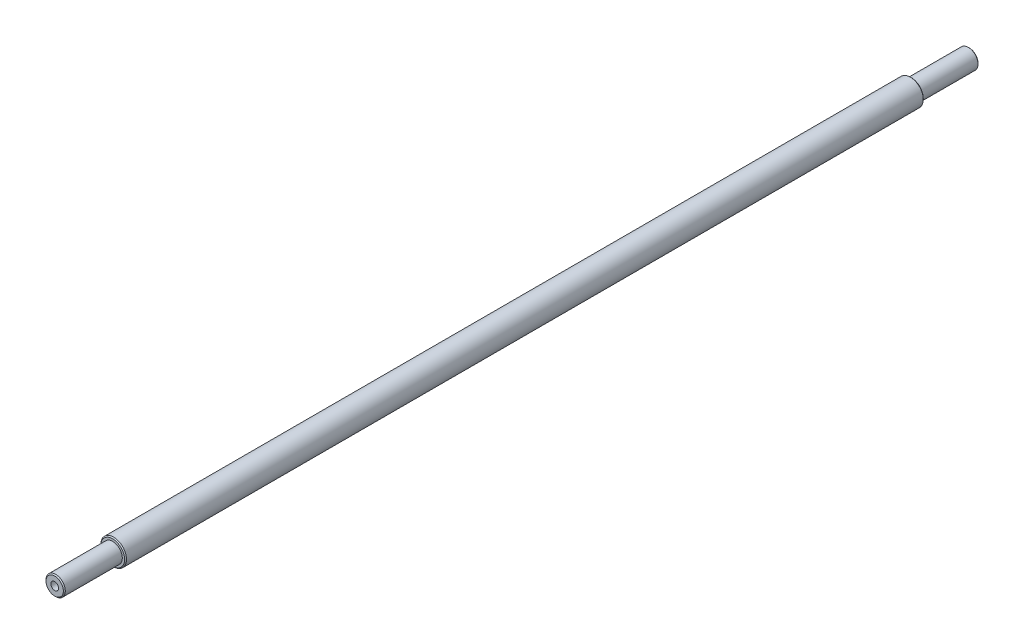
SolidWorks part; units mm, degrees
ref_plane "Front Plane" through (0, 0, 0) normal (0, 0, 1) x (1, 0, 0)
ref_plane "Top Plane" through (0, 0, 0) normal (0, 1, 0) x (1, 0, 0)
ref_plane "Right Plane" through (0, 0, 0) normal (1, 0, 0) x (0, 0, -1)
sketch "Sketch1" plane through (0, 0, 0) normal (0, 0, 1) x (1, 0, 0)
  circle A0 centre (0, 0) radius 15
  dimension "D1" = 30
extrude "Boss-Extrude1" add sketch "Sketch1" along normal mid plane 1420
hole_wizard "M14 Tapped Hole2" positions "Sketch3" profile "Sketch4" tap size "M14" standard "GB"
sketch "Sketch3" plane through (0, 0, 710) normal (0, 0, 1) x (1, 0, 0)
  point P0 (0, 0)
sketch "Sketch4" plane through (0, 0, 710) normal (1, 0, 0) x (0, -1, 0)
  line L0 (0, 0) -> (0, 37.6052)
  line L1 (0, 37.6052) -> (6, 34)
  line L2 (6, 34) -> (6, 0)
  line L5 (6, 0) -> (0, 0)
  line L10 (0, 37.6052) -> (-6, 34) construction
  line L11 (0, -6.35) -> (0, 107.95) construction
  dimension "螺纹孔钻头直径" = 12
  dimension "螺纹孔钻头深度" = 34
  dimension "导头角度" = 118
cosmetic thread "Cosmetic Thread1" parameters "D1"=28, "D2"=14
hole_wizard "M14 Tapped Hole1" positions "Sketch5" profile "Sketch6" tap size "M14" standard "GB"
sketch "Sketch5" plane through (0, 0, -710) normal (0, 0, -1) x (-1, 0, 0)
  point P0 (0, 0)
sketch "Sketch6" plane through (0, 0, -710) normal (1, 0, 0) x (0, 1, 0)
  line L0 (0, 0) -> (0, 37.6052)
  line L1 (0, 37.6052) -> (6, 34)
  line L2 (6, 34) -> (6, 0)
  line L5 (6, 0) -> (0, 0)
  line L10 (0, 37.6052) -> (-6, 34) construction
  line L11 (0, -6.35) -> (0, 107.95) construction
  dimension "螺纹孔钻头直径" = 12
  dimension "螺纹孔钻头深度" = 34
  dimension "导头角度" = 118
cosmetic thread "Cosmetic Thread2" parameters "D1"=28, "D2"=14
sketch "Sketch7" plane through (0, 0, 0) normal (0, 0, 1) x (1, 0, 0)
  circle A0 centre (0, 0) radius 20
  dimension "D1" = 40
extrude "Boss-Extrude3" add sketch "Sketch7" along normal mid plane 1240
chamfer "Chamfer1" distance 1.5 angle 45 4 edges at (15, 0, 710) (20, 0, 620) (20, 0, -620) (15, 0, -710)
